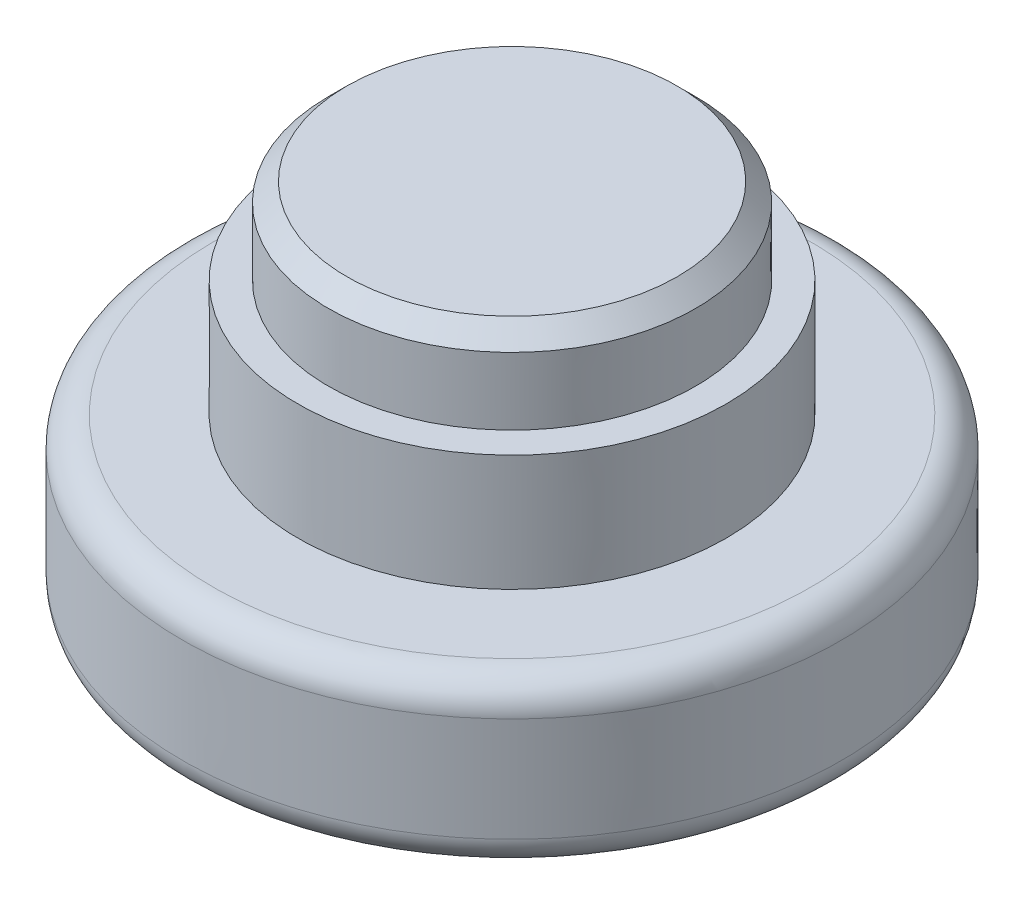
from build123d import *


with BuildPart() as part:
    # Sketch1 → Revolve1 (revolve)
    with BuildSketch(Plane.XY, mode=Mode.PRIVATE) as revolve1_sk:
        with BuildLine():
            Line((0, 0), (27, 0))
            Line((27, 0), (30, -3))
            Line((30, -3), (30, -14))
            Line((30, -14), (35, -14))
            Line((35, -14), (35, -33))
            Line((35, -33), (48.85, -33))
            ThreePointArc((48.85, -33), (52.385533906, -34.464466094), (53.85, -38))
            Line((53.85, -38), (53.85, -55.029219265))
            ThreePointArc((53.85, -55.029219265), (52.955142356, -57.883655503), (50.590877505, -59.716366106))
            Line((50.590877505, -59.716366106), (40.331108761, -63.527))
            Line((40.331108761, -63.527), (34.844391239, -63.527))
            Line((34.844391239, -63.527), (34.844391239, -64.4758))
            Line((34.844391239, -64.4758), (0.001691239, -64.4758))
            Line((0.001691239, -64.4758), (0, 0))
        make_face()
    revolve(revolve1_sk.sketch.rotate(Axis((0, 0, 0), (2.6230605830006534e-05, -0.9999999996559776, 0)), 180), axis=Axis((0, 0, 0), (2.6230605830006534e-05, -0.9999999996559776, 0)))


solid = part.part
